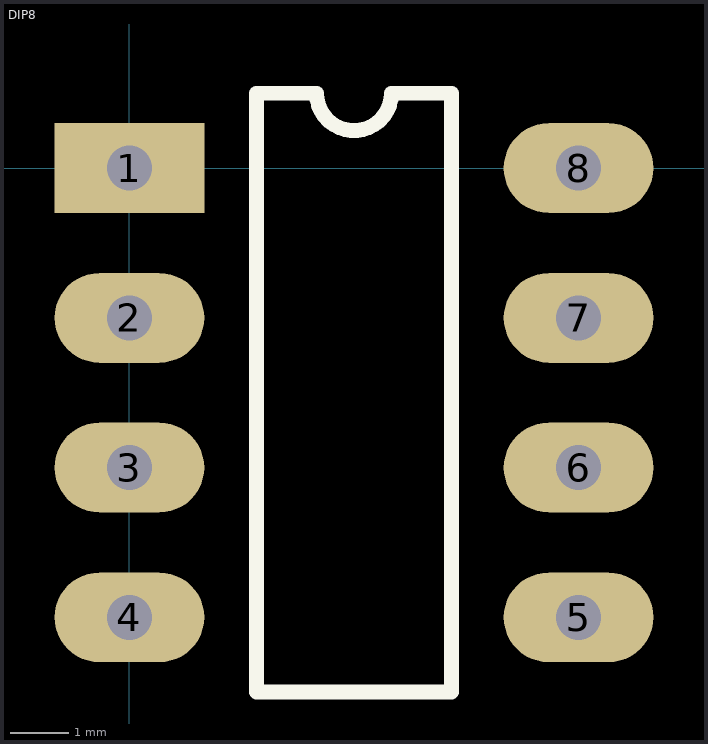
[diagram p0: the footprint, top view; thin cyan lines are the x and y axes]
# Altium footprint library MISC82778-2.PcbLib: 1 footprints
Each footprint in its own frame and in the unit in brackets; x right, y up, seen from the top. Pads: shape width x height; smd on the part's side, far side on the other; paste and mask are expansions set on the pad; w line width, h text height; cw(c..) or ccw(c..) is an arc to the next point about the centre after c.

## DIP8 [mil]
pads (8):
  rect 100x60 hole 30: 1(0,0)
  oval 100x60 hole 30: 2(0,-100) 3(0,-200) 4(0,-300) 5(300,-300) 6(300,-200) 7(300,-100) 8(300,0)
Top Overlay:
  lines w10: 85,-350 85,50 125,50 ccw(c150,50) 175,50 215,50 215,-350 85,-350